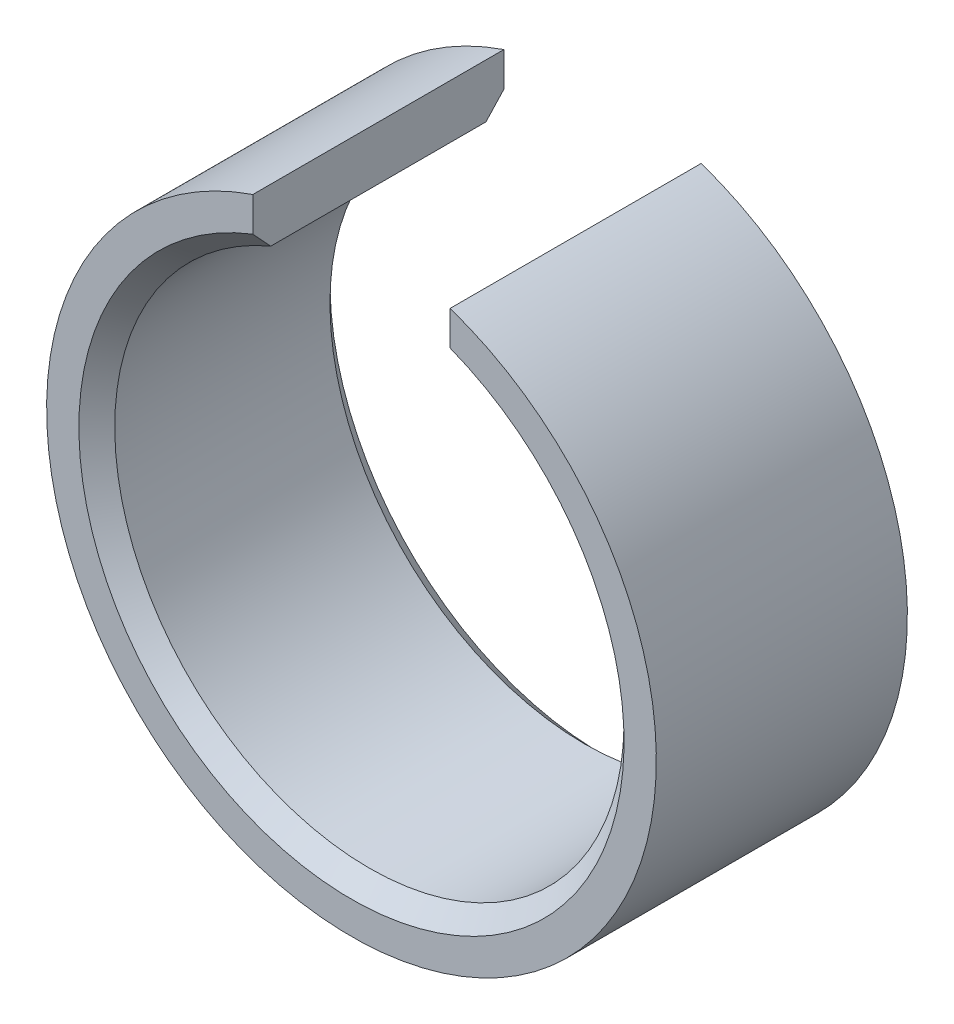
from build123d import *

# Parameters (mm, degrees)
SKETCH1_R           = 8.5
SKETCH1_R_2         = 7.1
BOSS_EXTRUDE1_DEPTH = 7
SKETCH2_W           = 5.5
SKETCH2_H           = 15
CUT_EXTRUDE1_DEPTH  = 14.910427743
CHAMFER1_SIZE       = 0.5


with BuildPart() as part:
    # Sketch1 → Boss-Extrude1 (new body)
    with BuildSketch(Plane.XY):
        Circle(SKETCH1_R)
        Circle(SKETCH1_R_2, mode=Mode.SUBTRACT)
    extrude(amount=BOSS_EXTRUDE1_DEPTH)

    # Sketch2 → Cut-Extrude1 (cut, through all)
    with BuildSketch(Plane.XY.offset(7)):
        with Locations((0, 7.5)):
            Rectangle(SKETCH2_W, SKETCH2_H)
    extrude(amount=-CUT_EXTRUDE1_DEPTH, mode=Mode.SUBTRACT)

    # Chamfer1
    chamfer1_edges = [part.edges().sort_by_distance(p)[0] for p in [
        (0, -7.1, 0),
        (0, -7.1, 7),
    ]]
    chamfer(chamfer1_edges, length=CHAMFER1_SIZE)


solid = part.part
